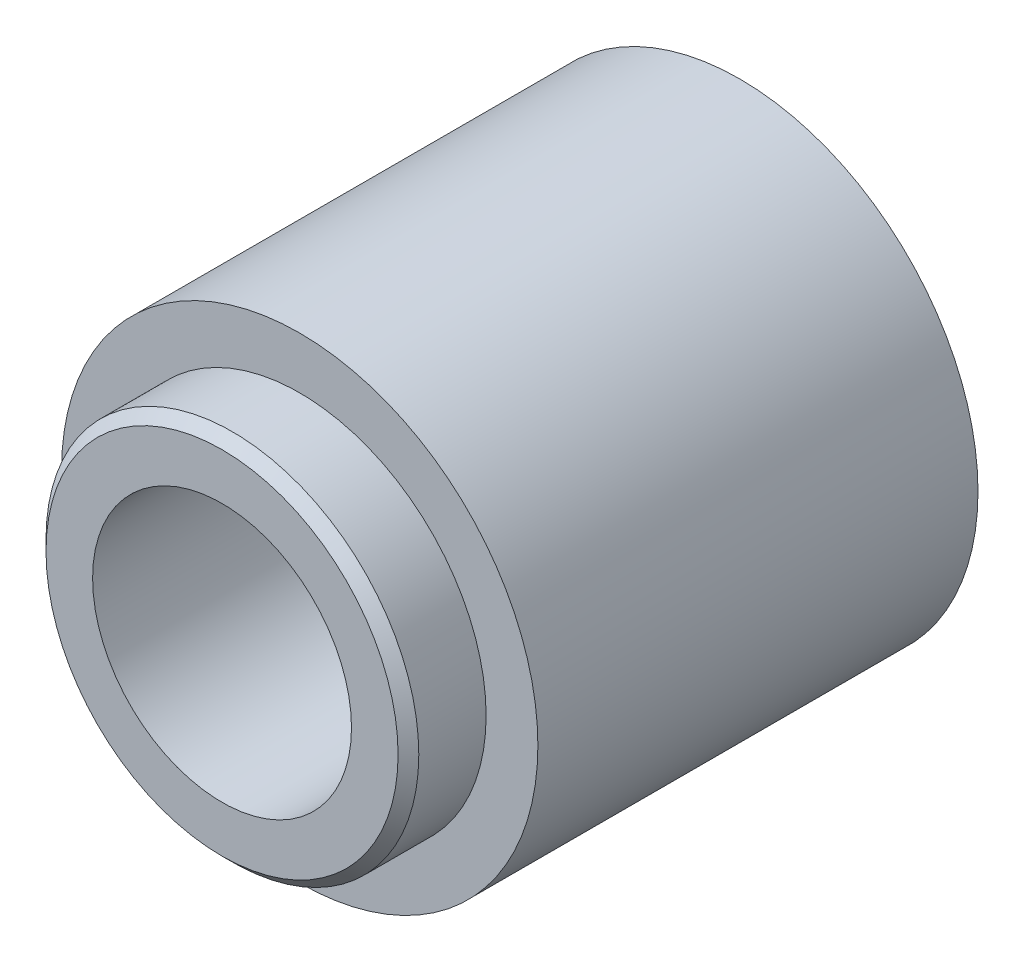
from build123d import *

# Parameters (mm, degrees)
SKETCH1_R           = 23
BOSS_EXTRUDE1_DEPTH = 50
CUT_EXTRUDE1_START  = -7.5
SKETCH2_R           = 23
SKETCH2_R_2         = 18
CUT_EXTRUDE1_DEPTH  = 7.5
SKETCH3_R           = 12.5
CUT_EXTRUDE2_DEPTH  = 60.648973168
CHAMFER1_SIZE       = 1


with BuildPart() as part:
    # Sketch1 → Boss-Extrude1 (new body)
    with BuildSketch(Plane.XY):
        Circle(SKETCH1_R)
    extrude(amount=BOSS_EXTRUDE1_DEPTH)

    # Sketch2 → Cut-Extrude1 (cut)
    with BuildSketch(Plane.XY.offset(50).offset(CUT_EXTRUDE1_START)):
        Circle(SKETCH2_R)
        Circle(SKETCH2_R_2, mode=Mode.SUBTRACT)
    extrude(amount=CUT_EXTRUDE1_DEPTH, mode=Mode.SUBTRACT)

    # Sketch3 → Cut-Extrude2 (cut, through all)
    with BuildSketch(Plane.XY.offset(50)):
        Circle(SKETCH3_R)
    extrude(amount=-CUT_EXTRUDE2_DEPTH, mode=Mode.SUBTRACT)

    # Chamfer1
    chamfer1_edges = [part.edges().sort_by_distance(p)[0] for p in [
        (-18, 0, 50),
    ]]
    chamfer(chamfer1_edges, length=CHAMFER1_SIZE)


solid = part.part
